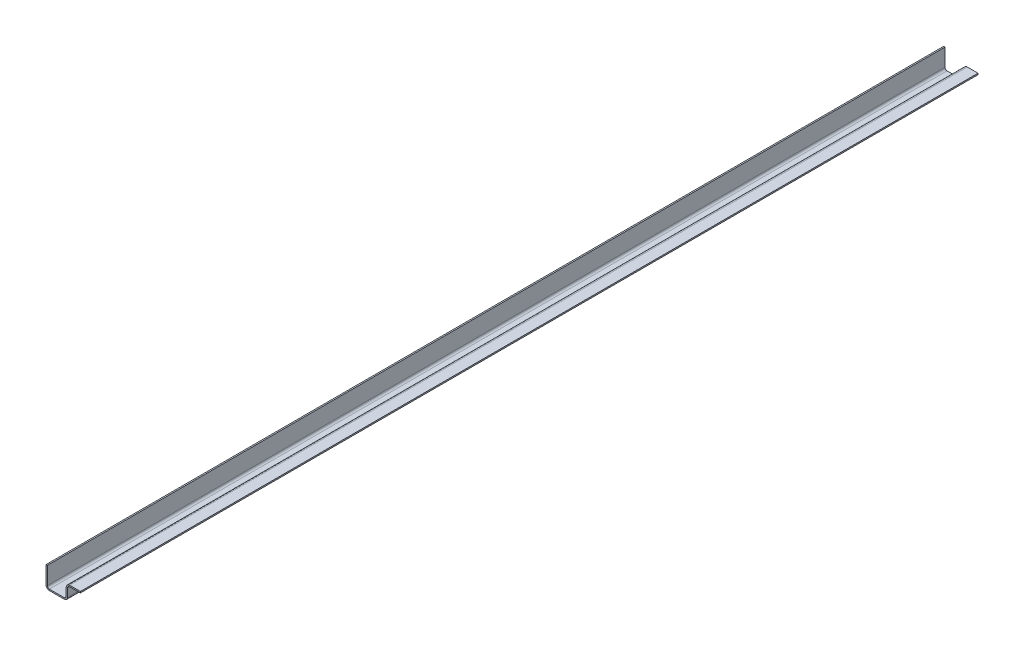
SolidWorks part; units mm, degrees
ref_plane "前视基准面" through (0, 0, 0) normal (0, 0, 1) x (1, 0, 0)
ref_plane "上视基准面" through (0, 0, 0) normal (0, 1, 0) x (1, 0, 0)
ref_plane "右视基准面" through (0, 0, 0) normal (1, 0, 0) x (0, 0, -1)
sketch "草图1" plane through (0, 0, 0) normal (0, 0, 1) x (1, 0, 0)
  line L0 (0, 30) -> (0, 0)
  line L1 (0, 0) -> (30, 0)
  line L2 (30, 0) -> (30, 20)
  line L3 (30, 20) -> (50, 20)
  dimension "D1" = 30
  dimension "D2" = 30
  dimension "D3" = 20
  dimension "D4" = 20
extrude "拉伸-薄壁1" add sketch "草图1" along normal mid plane 1331 thin thin type mid plane wall 2
